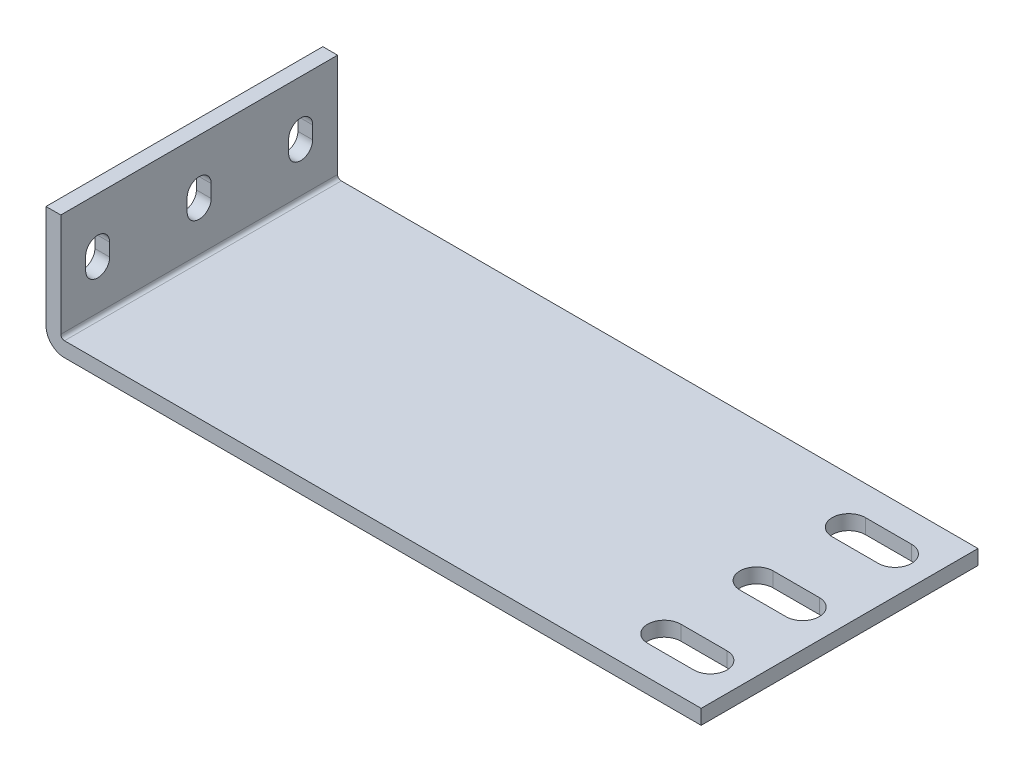
SolidWorks part; units mm, degrees
material "1023 碳钢板 (SS)"
ref_plane "前视基准面" through (0, 0, 0) normal (0, 0, 1) x (1, 0, 0)
ref_plane "上视基准面" through (0, 0, 0) normal (0, 1, 0) x (1, 0, 0)
ref_plane "右视基准面" through (0, 0, 0) normal (1, 0, 0) x (0, 0, -1)
sketch "草图1" plane through (0, 0, 0) normal (0, 0, 1) x (1, 0, 0)
  line L0 (0, 0) -> (0, -56)
  line L1 (10, -66) -> (355, -66)
  line L2 (8, 0) -> (8, -56)
  line L3 (10, -58) -> (355, -58)
  line L4 (8, 0) -> (0, 0)
  line L5 (355, -58) -> (355, -66)
  arc A0 (0, -56) -> (10, -66) centre (10, -56) ccw
  arc A1 (8, -56) -> (10, -58) centre (10, -56) ccw
  point P6 (0, -66)
  dimension "D3" = 10
  dimension "D1" = 66
  dimension "D2" = 355
  dimension "D4" = 8
extrude "凸台-拉伸1" add sketch "草图1" along normal blind 150
sketch "草图2" plane through (0, 0, 0) normal (-1, 0, 0) x (0, 0, 1)
  line L0 (20, -26) -> (20, -33) construction
  line L1 (26.5, -26) -> (26.5, -33)
  line L2 (13.5, -26) -> (13.5, -33)
  line L3 (75, -26) -> (75, -33) construction
  line L4 (81.5, -26) -> (81.5, -33)
  line L5 (68.5, -26) -> (68.5, -33)
  line L6 (130, -26) -> (130, -33) construction
  line L7 (136.5, -26) -> (136.5, -33)
  line L8 (123.5, -26) -> (123.5, -33)
  line L9 (0, 0) -> (0, -56) construction
  line L10 (150, -66) -> (0, -66) construction
  arc A0 (26.5, -26) -> (13.5, -26) centre (20, -26) ccw
  arc A1 (13.5, -33) -> (26.5, -33) centre (20, -33) ccw
  arc A2 (81.5, -26) -> (68.5, -26) centre (75, -26) ccw
  arc A3 (68.5, -33) -> (81.5, -33) centre (75, -33) ccw
  arc A4 (136.5, -26) -> (123.5, -26) centre (130, -26) ccw
  arc A5 (123.5, -33) -> (136.5, -33) centre (130, -33) ccw
  point P2 (20, -29.5)
  point P7 (75, -29.5)
  point P14 (130, -29.5)
  point P25 (0, 0)
  dimension "D4" = 6.5
  dimension "D1" = 55
  dimension "D2" = 55
  dimension "D3" = 7
  dimension "D5" = 20
  dimension "D6" = 36.5
extrude "切除-拉伸1" cut sketch "草图2" against normal blind 150
sketch "草图3" plane through (0, -58, 0) normal (0, 1, 0) x (1, 0, 0)
  line L0 (310, -25) -> (335, -25) construction
  line L1 (310, -16) -> (335, -16)
  line L2 (310, -34) -> (335, -34)
  line L3 (310, -75) -> (335, -75) construction
  line L4 (310, -66) -> (335, -66)
  line L5 (310, -84) -> (335, -84)
  line L6 (310, -125) -> (335, -125) construction
  line L7 (310, -116) -> (335, -116)
  line L8 (310, -134) -> (335, -134)
  line L9 (355, 0) -> (10, 0) construction
  line L10 (355, -150) -> (355, 0) construction
  arc A0 (310, -16) -> (310, -34) centre (310, -25) ccw
  arc A1 (335, -34) -> (335, -16) centre (335, -25) ccw
  arc A2 (310, -66) -> (310, -84) centre (310, -75) ccw
  arc A3 (335, -84) -> (335, -66) centre (335, -75) ccw
  arc A4 (310, -116) -> (310, -134) centre (310, -125) ccw
  arc A5 (335, -134) -> (335, -116) centre (335, -125) ccw
  point P2 (322.5, -25)
  point P7 (322.5, -75)
  point P14 (322.5, -125)
  point P25 (0, 0)
  dimension "D5" = 9
  dimension "D6" = 20
  dimension "D1" = 25
  dimension "D2" = 50
  dimension "D3" = 50
  dimension "D4" = 25
extrude "切除-拉伸2" cut sketch "草图3" against normal blind 150
